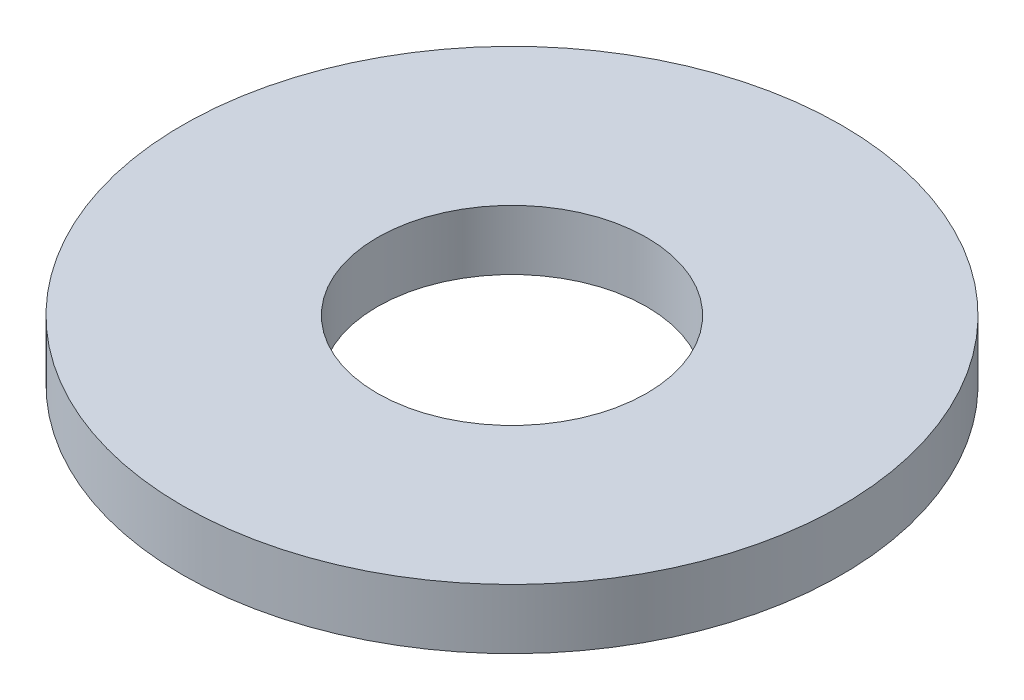
from build123d import *

# Parameters (mm, degrees)
SKETCH_1_R      = 110
SKETCH_1_R_2    = 45
EXTRUDE_1_DEPTH = 20


with BuildPart() as part:
    # 草图1 → 凸台-拉伸1 (new body)
    with BuildSketch(Plane(origin=(0, 0, 0), x_dir=(1, 0, 0), z_dir=(0, 1, 0))):
        with Locations(Location((0, 0, 0), (0, 0, 270))):
            Circle(SKETCH_1_R)
        with Locations(Location((0, 0, 0), (0, 0, 270))):
            Circle(SKETCH_1_R_2, mode=Mode.SUBTRACT)
    extrude(amount=EXTRUDE_1_DEPTH)


solid = part.part
